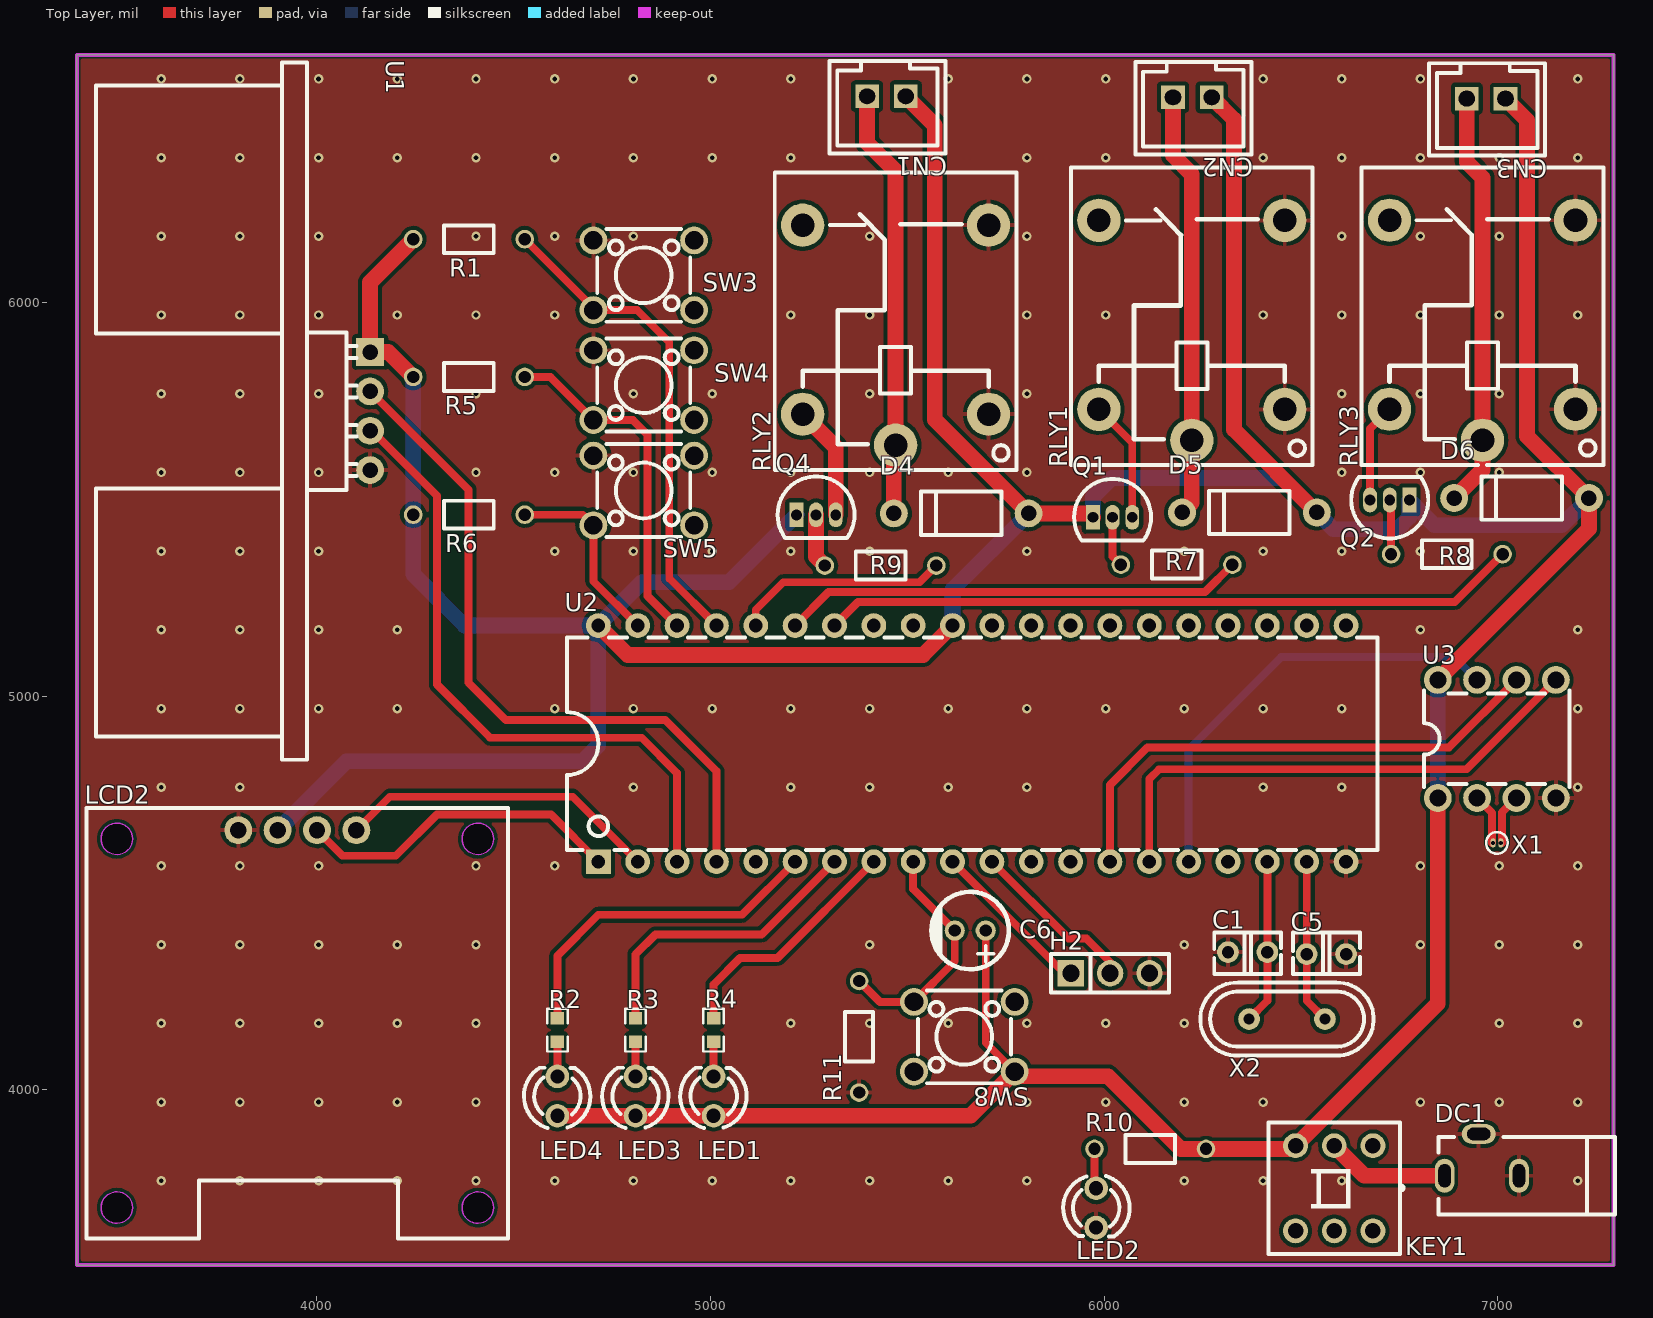
[diagram p0: Top Layer view]
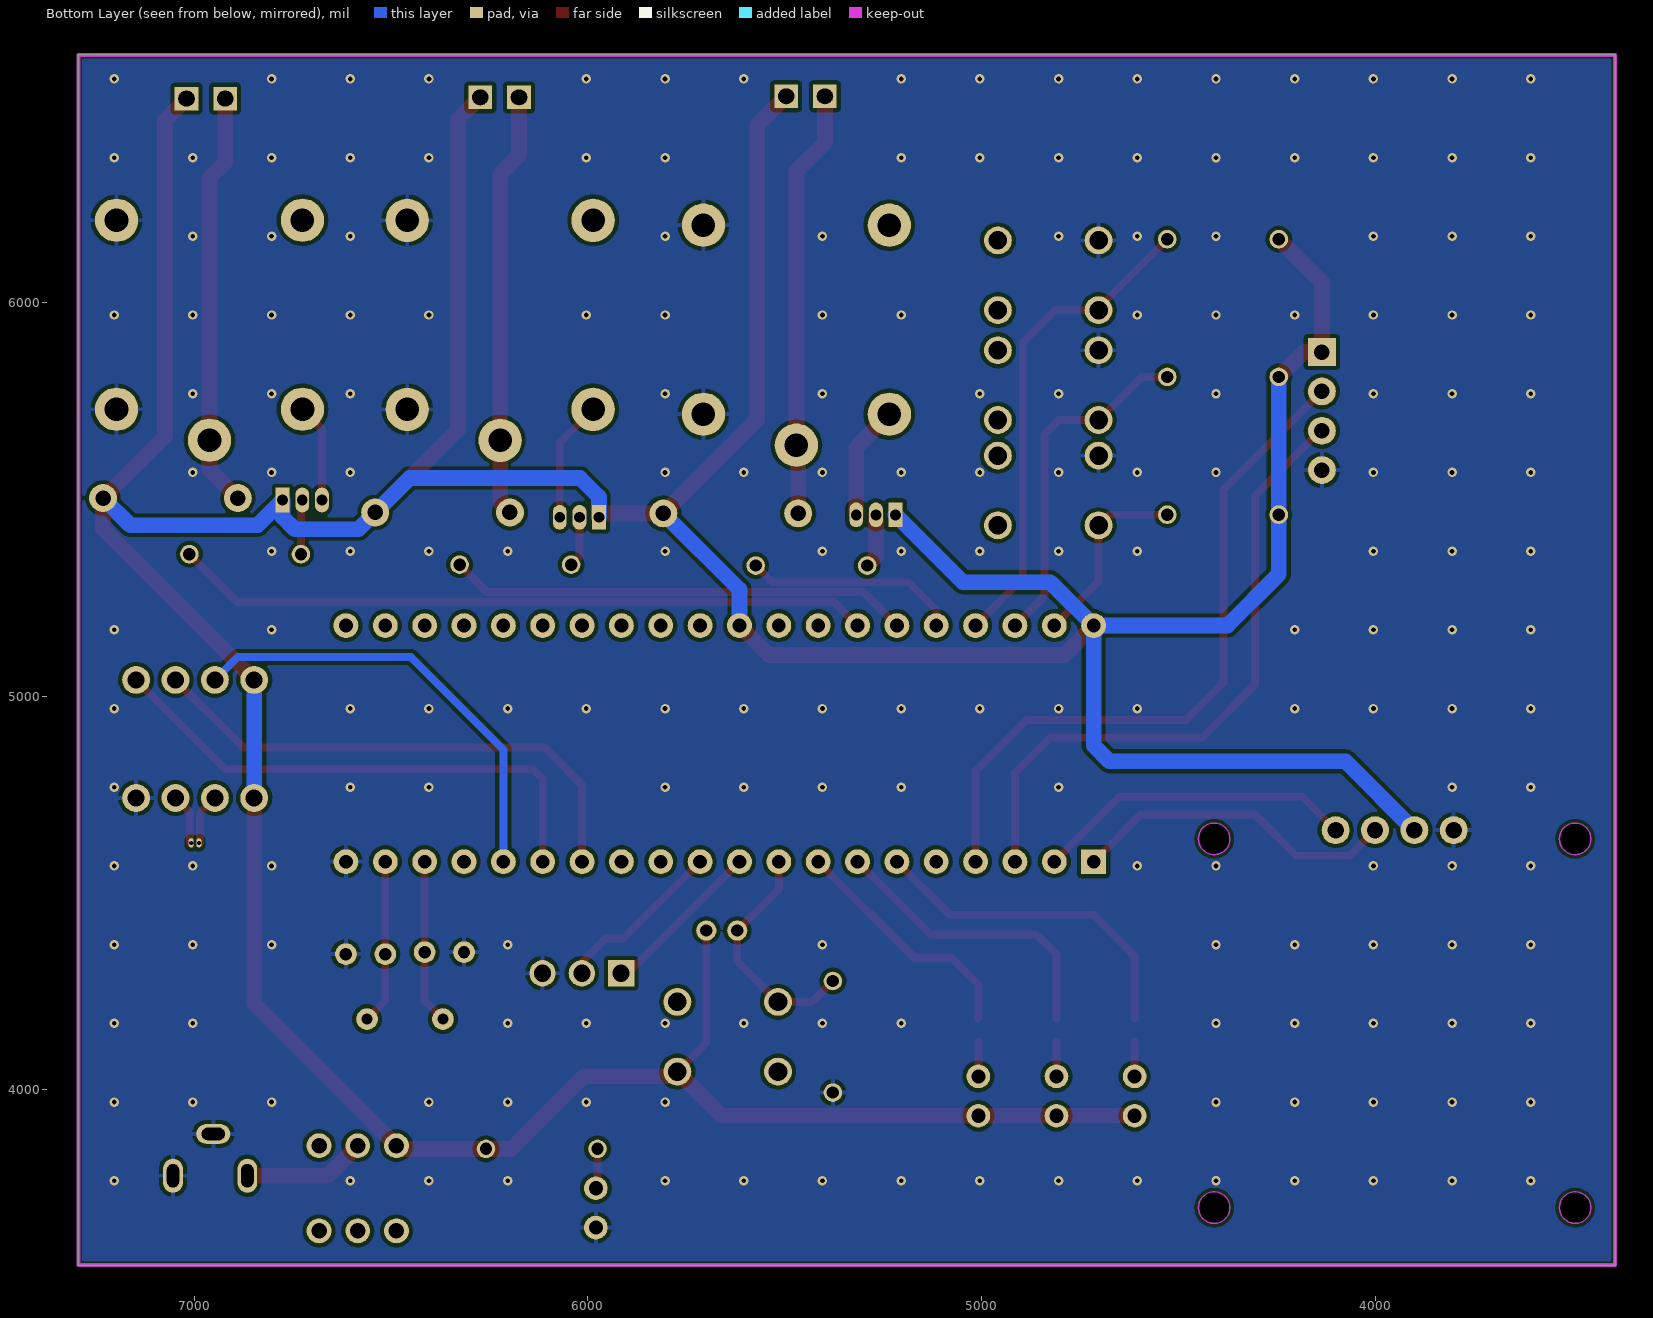
[diagram p1: Bottom Layer view, seen from below]
# Altium PCB MISC52010.pcbdoc
Units mil, origin at the board's own origin, x right, y up, seen from the top; angles counter-clockwise.
Board outline 3905 x 3075 mil, 2 copper layers (Top Layer, Bottom Layer), stack 62.206 mil thick; 43 components, 39 nets, 160 pads, 187 vias.

## Layer stack, top to bottom
Top Solder Mask Layer: solder mask 0.394, Dk 3.3
Top Layer: signal copper 1.379
Dielectric1: surface 59.449, FR4, Dk 4.5
Bottom Layer: signal copper 1.378
Bottom Solder Mask Layer: solder mask 0.394, Dk 3.3

## Board outline
3390,6630 3390,3555 7295,3555 7295,6630

## Design rules (kind name [scope] priority, off if disabled: settings)
BoardOutlineClearance copperThickness2oz_1 [All] p2 off: genericclearance=7.99 ignorepadtopadclearanceinfootprint=FALSE except(0: Arc-SplitContinuation Track-SplitContinuation SMDPad-SplitContinuation THPad-SplitContinuation Via-SplitContinuation Fill-SplitContinuation Region-SplitContinuation Poly-SplitContinuation Text-SplitContinuation Hole-SplitContinuation; 5.98: Arc-CutoutEdge SMDPad-CutoutEdge THPad-CutoutEdge Via-CutoutEdge Fill-CutoutEdge Region-CutoutEdge Text-CutoutEdge; 6.93: Hole-OutlineEdge Hole-CutoutEdge; 10: Poly-OutlineEdge Poly-CutoutEdge; 11.81: Arc-OutlineEdge Track-OutlineEdge SMDPad-OutlineEdge THPad-OutlineEdge Via-OutlineEdge Fill-OutlineEdge Region-OutlineEdge Text-OutlineEdge Track-CutoutEdge)
BoardOutlineClearance copperThickness1oz_1 [All] p4: genericclearance=4.02 ignorepadtopadclearanceinfootprint=FALSE except(0: Arc-SplitContinuation Track-SplitContinuation SMDPad-SplitContinuation THPad-SplitContinuation Via-SplitContinuation Fill-SplitContinuation Region-SplitContinuation Poly-SplitContinuation Text-SplitContinuation Hole-SplitContinuation; 6: SMDPad-CutoutEdge THPad-CutoutEdge Via-CutoutEdge Fill-CutoutEdge Region-CutoutEdge Text-CutoutEdge; 6.93: Hole-OutlineEdge Hole-CutoutEdge; 10: Poly-OutlineEdge Poly-CutoutEdge; 11.8: Arc-OutlineEdge Track-OutlineEdge SMDPad-OutlineEdge THPad-OutlineEdge Via-OutlineEdge Fill-OutlineEdge Region-OutlineEdge Text-OutlineEdge; 11.81: Arc-CutoutEdge Track-CutoutEdge)
Clearance copperThickness2oz [All] p1 off: gap=7.99 ignorepadtopadclearanceinfootprint=FALSE except(5.98: SMDPad-Track SMDPad-SMDPad THPad-Track SMDPad-THPad THPad-THPad Track-Via SMDPad-Via THPad-Via Via-Via Fill-Track Region-Track Fill-SMDPad Region-SMDPad Fill-THPad Region-THPad Fill-Via Region-Via Fill-Fill Fill-Region Region-Region Arc-Track Arc-SMDPad Arc-THPad Arc-Via Fill-Arc Region-Arc Arc-Arc Text-Track SMDPad-Text Text-THPad Text-Via Fill-Text Region-Text Arc-Text Text-Text; 6.93: Hole-Track Hole-SMDPad Hole-THPad Hole-Via Fill-Hole Region-Hole Hole-Arc Hole-Text; 10: Poly-Track Poly-SMDPad Poly-THPad Poly-Via Poly-Fill Poly-Region Poly-Poly Poly-Arc Poly-Text Poly-Hole)
Clearance copperThickness1oz [All] p3: gap=4.02 ignorepadtopadclearanceinfootprint=FALSE except(5.98: SMDPad-Track SMDPad-SMDPad THPad-Track SMDPad-THPad THPad-THPad Track-Via SMDPad-Via THPad-Via Via-Via Fill-Track Region-Track Fill-SMDPad Region-SMDPad Fill-THPad Region-THPad Fill-Via Region-Via Fill-Fill Fill-Region Region-Region; 6: Arc-Track Arc-SMDPad Arc-THPad Arc-Via Fill-Arc Region-Arc Arc-Arc Text-Track SMDPad-Text Text-THPad Text-Via Fill-Text Region-Text Arc-Text Text-Text; 6.93: Hole-Track Hole-SMDPad Hole-THPad Hole-Via Fill-Hole Region-Hole Hole-Arc Hole-Text; 10: Poly-Track Poly-SMDPad Poly-THPad Poly-Via Poly-Fill Poly-Region Poly-Poly Poly-Arc Poly-Text Poly-Hole)
Creepage creepage [All] p1: checkdistance=0 ignoreinternallayers=TRUE applytopolygonpour=TRUE
DiffPairsRouting differentialPair [All] p1: maxlimit=6 minlimit=6 mostfreqgap=6 toplayer_minwidth=5 toplayer_prefwidth=10 toplayer_maxwidth=100 toplayer_mingap=6 toplayer_prefgap=6 toplayer_maxgap=6 bottomlayer_minwidth=5 bottomlayer_prefwidth=10 bottomlayer_maxwidth=100 bottomlayer_mingap=6 bottomlayer_prefgap=6 bottomlayer_maxgap=6 maxuncoupledlength=10
HoleToHoleClearance otherClearance [All] p1: gap=11.81 allowstackedmicrovias=TRUE
Length netLength [All] p1: minlimit=0 maxlimit=0
MatchedLengths netLengthTolerance [All] p1: tolerance=1000
PasteMaskExpansion pasteMaskExpansion [All] p1: expansion=0
PlaneConnect innerPlane [All] p1: planeconnectstyle=Relief reliefexpansion=20 reliefentries=4 reliefconductorwidth=10 reliefairgap=10
PolygonConnect copperRegion [(InNet('GND'))] p1: connectstyle=Relief reliefconductorwidth=10 reliefentries=4 polygonreliefangle="90 Angle" airgapwidth=10 via.connectstyle=Relief via.reliefconductorwidth=10 via.reliefentries=4 via.polygonreliefangle="90 Angle" via.airgapwidth=10
RoutingVias viaSize [All] p1: holewidth=12.01 width=24.02 viastyle="Through Hole" minholewidth=11.81 minwidth=19.68 maxholewidth=248.03 maxwidth=393.7
SolderMaskExpansion solderMaskExpansion [IsVia] p1: expansion=-1000 istentingtop=TRUE
SolderMaskExpansion solderMaskExpansion [All] p2: expansion=2 istentingtop=FALSE
Width copperThickness2oz_2 [All] p1 off: maxlimit=100 minlimit=8 preferedwidth=10
Width copperThickness1oz_2 [All] p2: maxlimit=100 minlimit=5 preferedwidth=10

## Components (designator, comment, footprint, x,y, rotation, side; value= is the part's Value field where it differs from the comment)
C1 "30pF" CAP-TH_L3.8-W2.5-P2.54-D0.50 6365,4350 r0 top
C5 "30pF" CAP-TH_L3.8-W2.5-P2.54-D0.50 6565,4345 r180 top
C6 "10uF" CAP-TH_BD5.0-P2.00-D0.8-FD-10UF50VC110GL 5660,4405 r180 top
CN1 "XH2.54-2PIN-直针" CONN-TH_XH2.54-2P 5447.09,6525.02 r180 top
CN2 "XH2.54-2PIN-直针" CONN-TH_XH2.54-2P 6224.43,6522.35 r180 top
CN3 "XH2.54-2PIN-直针" CONN-TH_XH2.54-2P 6971.03,6518.96 r180 top
D4 "" DO_1N4007 5637.09,5465.02 r0 top
D5 "" DO_1N4007 6369.43,5467.35 r0 top
D6 "" DO_1N4007 7061.03,5503.96 r0 top
DC1 "DC-002" DC-IN-TH_DC-3510 6960,3835 r0 top
H2 "" HDR-TH_3P-P2.54-V-M 6015.53,4296.39 r0 top
KEY1 "无自锁开关 8.5×8.5 无声" SW-TH_6P-L8.5-W8.5-P2.54 6585,3750 r180 top
LCD2 "HS96L03W2C03" OLED-TH_L27.8-W27.2-P2.54_C9900033791 3950,4660 r0 top
LED1 "" LED_TH-3mm 5007.91,3984.24 r90 top
LED2 "" LED_TH-3mm 5980,3700 r270 top
LED3 "" LED_TH-3mm 4809.41,3984.24 r90 top
LED4 "" LED_TH-3mm 4610.91,3984.24 r90 top
Q1 "" S8550P_TO-92 6021.71,5455.16 r0 top
Q2 "" S8550P_TO-92 6726.03,5498.96 r180 top
Q4 "" S8550P_TO-92 5268.28,5461.34 r0 top
R1 "10kΩ" Res_1/8W 4386.23,6164.19 r180 top
R2 "220" R0603 4610.91,4152.03 r90 top
R3 "220" R0603 4809.41,4152.03 r90 top
R4 "220" R0603 5007.91,4152.03 r90 top
R5 "10kΩ" Res_1/8W 4386.23,5814.19 r180 top
R6 "10kΩ" Res_1/8W 4386.23,5464.19 r180 top
R7 "1kΩ" Res_1/8W 6184.43,5332.35 r0 top
R8 "1kΩ" Res_1/8W 6871.03,5358.96 r0 top
R9 "1kΩ" Res_1/8W 5432.09,5330.02 r0 top
R10 "1kΩ" Res_1/8W 6117.48,3847.52 r0 top
R11 "10kΩ" Res_1/8W 5380,4135 r90 top
RLY1 "SRD-05VDC-SL-C" RELAY-TH_SRD-XXVDC-XL-C 6223.04,5930.16 r90 top
RLY2 "SRD-05VDC-SL-C" RELAY-TH_SRD-XXVDC-XL-C 5470.38,5917.82 r90 top
RLY3 "SRD-05VDC-SL-C" RELAY-TH_SRD-XXVDC-XL-C 6961.75,5930.43 r90 top
SW3 "" SW-TH_4P-L6.0-W6.0-P4.50-LS6.5 4830.32,6070.09 r180 top
SW4 "" SW-TH_4P-L6.0-W6.0-P4.50-LS6.5 4830.32,5790.96 r180 top
SW5 "" SW-TH_4P-L6.0-W6.0-P4.50-LS6.5 4830.32,5523.25 r180 top
SW8 "" SW-TH_4P-L6.0-W6.0-P4.50-LS6.5 5645,4135 r180 top
U1 "HC-SR04" TH_HC-SR04V 4135,5725 r270 top
U2 "STC89C52RC-40I-PDIP40" DIP-40_L52.0-W13.7-P2.54-LS15.2-BL 5665,4880 r0 top
U3 "DS1302N(XBLW)" PDIP-8_L9.3-W6.4-P2.54-LS7.6-BL 6998.11,4891.89 r0 top
X1 "32.768kHz" CRYSTAL-TH_BD1.4-P0.45-D0.2 6998.47,4627.72 r180 top
X2 "11.0592MHz" OSC-TH_L11.1-W4.7-P4.88 6465,4180 r180 top

## Footprints (in the part's own frame and the unit in brackets; to place one, negate y for a bottom-side part, rotate by r counter-clockwise, add the part's x,y. Pads: shape width x height; smd on the part's side, far side on the other; paste and mask are expansions set on the pad)
CAP-TH_BD5.0-P2.00-D0.8-FD-10UF50VC110GL [mm]
  round 1.3 hole 0.8: 1(-1,0) 2(1,0)
  silkscreen extent -2.5,-2.5 2.5,2.5
CAP-TH_L3.8-W2.5-P2.54-D0.50 [mm]
  round 1.4 hole 0.8 paste+0 mask+0.05: 1(-1.27,0) 2(1.27,0)
  silkscreen extent -2.16,-1.4 2.16,1.27
CONN-TH_XH2.54-2P [mil]
  rect 60x60 hole 39.37 slot 41.34 at 0 deg paste+0 mask+1.97: 1(-49.22,0) 2(49.21,0)
  silkscreen extent -150,-90 145,145
CRYSTAL-TH_BD1.4-P0.45-D0.2 [mm]
  oval 0.32x0.6 hole 0.27 paste+0 mask+0.05: 1(-0.25,0) 2(0.25,0)
  silkscreen extent -0.7,-0.7 0.7,0.7
DC-IN-TH_DC-3510 [mm]
  oval 1.27x2.2 hole 0.8 slot 1.5 at 90 deg: 1(-2.4,-1.35) 2(2.4,-1.35)
  oval 2.2x1.27 hole 0.8 slot 1.5 at 0 deg: 3(-0.2,1.35)
  silkscreen extent -2.8,-3.85 8.6,1.15
DIP-40_L52.0-W13.7-P2.54-LS15.2-BL [mil]
  rect 63x63 hole 35: 1(-950,-300)
  round 63 hole 35: 2(-850,-300) 3(-750,-300) 4(-650,-300) 5(-550,-300) 6(-450,-300) 7(-350,-300) 8(-250,-300) 9(-150,-300) 10(-50,-300) 11(50,-300) 12(150,-300) 13(250,-300) 14(350,-300) 15(450,-300) 16(550,-300) 17(650,-300) 18(750,-300) 19(850,-300) 20(950,-300) 21(950,300) 22(850,300) 23(750,300) 24(650,300) 25(550,300) 26(450,300) 27(350,300) 28(250,300) 29(150,300) 30(50,300) 31(-50,300) 32(-150,300) 33(-250,300) 34(-350,300) 35(-450,300) 36(-550,300) 37(-650,300) 38(-750,300) 39(-850,300) 40(-950,300)
  silkscreen extent -1030,-270 1030,270
DO_1N4007 [mm]
  round 1.8 hole 1 paste+0 mask+0.051: 1(-4.35,0) 2(4.35,0)
  silkscreen extent -2.6,-1.4 2.6,1.4
HDR-TH_3P-P2.54-V-M [mm]
  rect 1.7x1.7 hole 1.1: 1(-2.54,0)
  round 1.7 hole 1.1: 2(0,0) 3(2.54,0)
  silkscreen extent -3.81,-1.25 3.81,1.25
LED_TH-3mm [mil]
  round 60 hole 36 paste+0 mask+2: 1(-50,0) 2(50,0)
  silkscreen extent -81,-84 72,85
OLED-TH_L27.8-W27.2-P2.54_C9900033791 [mm]
  round 1.8 hole 1.05 paste+0 mask+0.05: 1(-3.81,0) 2(-1.27,0) 3(1.27,0) 4(3.81,0)
  Board Outline Layer circle w0.003: c-11.65,-0.56 r1.016
  Board Outline Layer circle w0.003: c11.65,-0.56 r1.016
  Board Outline Layer circle w0.003: c-11.65,-24.36 r1.016
  Board Outline Layer circle w0.003: c11.65,-24.36 r1.016
  Board Outline Layer region: -10.634,-0.56 -10.735,-1.001 -11.016,-1.354 -11.424,-1.551 -11.876,-1.551 -12.283,-1.354 -12.565,-1.001 -12.666,-0.56 -12.666,-0.56 -12.565,-0.119 -12.283,0.234 -11.876,0.431 -11.424,0.431 -11.016,0.234 -10.735,-0.119 -10.634,-0.56
  Board Outline Layer region: -10.634,-0.56 -10.643,-0.698 -10.672,-0.834 -10.718,-0.965 -10.782,-1.088 -10.862,-1.201 -10.956,-1.303 -11.064,-1.39 -11.183,-1.462 -11.31,-1.517 -11.443,-1.555 -11.581,-1.574 -11.719,-1.574 -11.857,-1.555 -11.99,-1.517 -12.117,-1.462 -12.236,-1.39 -12.343,-1.303 -12.438,-1.201 -12.518,-1.088 -12.582,-0.965 -12.628,-0.834 -12.656,-0.698 -12.666,-0.56 -12.656,-0.422 -12.628,-0.286 -12.582,-0.155 -12.518,-0.032 -12.438,0.081 -12.343,0.183 -12.236,0.27 -12.117,0.342 -11.99,0.397 -11.857,0.435 -11.719,0.454 -11.581,0.454 -11.443,0.435 -11.31,0.397 -11.183,0.342 -11.064,0.27 -10.956,0.183 -10.862,0.081 -10.782,-0.032 -10.718,-0.155 -10.672,-0.286 -10.643,-0.422
  Board Outline Layer region: 12.666,-0.56 12.565,-1.001 12.283,-1.354 11.876,-1.551 11.424,-1.551 11.017,-1.354 10.735,-1.001 10.634,-0.56 10.634,-0.56 10.735,-0.119 11.017,0.234 11.424,0.431 11.876,0.431 12.283,0.234 12.565,-0.119 12.666,-0.56
  Board Outline Layer region: 12.666,-0.56 12.657,-0.698 12.628,-0.834 12.582,-0.965 12.518,-1.088 12.438,-1.201 12.343,-1.303 12.236,-1.39 12.117,-1.462 11.99,-1.517 11.857,-1.555 11.719,-1.574 11.581,-1.574 11.443,-1.555 11.31,-1.517 11.183,-1.462 11.064,-1.39 10.957,-1.303 10.862,-1.201 10.782,-1.088 10.718,-0.965 10.672,-0.834 10.643,-0.698 10.634,-0.56 10.643,-0.422 10.672,-0.286 10.718,-0.155 10.782,-0.032 10.862,0.081 10.957,0.183 11.064,0.27 11.183,0.342 11.31,0.397 11.443,0.435 11.581,0.454 11.719,0.454 11.857,0.435 11.99,0.397 12.117,0.342 12.236,0.27 12.343,0.183 12.438,0.081 12.518,-0.032 12.582,-0.155 12.628,-0.286 12.657,-0.422
  Board Outline Layer region: -10.634,-24.36 -10.735,-24.801 -11.016,-25.154 -11.424,-25.35 -11.876,-25.35 -12.283,-25.154 -12.565,-24.801 -12.666,-24.36 -12.666,-24.36 -12.565,-23.919 -12.283,-23.566 -11.876,-23.369 -11.424,-23.369 -11.016,-23.566 -10.735,-23.919 -10.634,-24.36
  Board Outline Layer region: -10.634,-24.36 -10.643,-24.498 -10.672,-24.634 -10.718,-24.765 -10.782,-24.888 -10.862,-25.001 -10.956,-25.102 -11.064,-25.19 -11.183,-25.262 -11.31,-25.317 -11.443,-25.355 -11.581,-25.374 -11.719,-25.374 -11.857,-25.355 -11.99,-25.317 -12.117,-25.262 -12.236,-25.19 -12.343,-25.102 -12.438,-25.001 -12.518,-24.888 -12.582,-24.765 -12.628,-24.634 -12.656,-24.498 -12.666,-24.36 -12.656,-24.222 -12.628,-24.086 -12.582,-23.955 -12.518,-23.832 -12.438,-23.719 -12.343,-23.617 -12.236,-23.53 -12.117,-23.458 -11.99,-23.403 -11.857,-23.365 -11.719,-23.346 -11.581,-23.346 -11.443,-23.365 -11.31,-23.403 -11.183,-23.458 -11.064,-23.53 -10.956,-23.617 -10.862,-23.719 -10.782,-23.832 -10.718,-23.955 -10.672,-24.086 -10.643,-24.222
  Board Outline Layer region: 12.666,-24.36 12.565,-24.801 12.283,-25.154 11.876,-25.35 11.424,-25.35 11.017,-25.154 10.735,-24.801 10.634,-24.36 10.634,-24.36 10.735,-23.919 11.017,-23.566 11.424,-23.369 11.876,-23.369 12.283,-23.566 12.565,-23.919 12.666,-24.36
  Board Outline Layer region: 12.666,-24.36 12.657,-24.498 12.628,-24.634 12.582,-24.765 12.518,-24.888 12.438,-25.001 12.343,-25.102 12.236,-25.19 12.117,-25.262 11.99,-25.317 11.857,-25.355 11.719,-25.374 11.581,-25.374 11.443,-25.355 11.31,-25.317 11.183,-25.262 11.064,-25.19 10.957,-25.102 10.862,-25.001 10.782,-24.888 10.718,-24.765 10.672,-24.634 10.643,-24.498 10.634,-24.36 10.643,-24.222 10.672,-24.086 10.718,-23.955 10.782,-23.832 10.862,-23.719 10.957,-23.617 11.064,-23.53 11.183,-23.458 11.31,-23.403 11.443,-23.365 11.581,-23.346 11.719,-23.346 11.857,-23.365 11.99,-23.403 12.117,-23.458 12.236,-23.53 12.343,-23.617 12.438,-23.719 12.518,-23.832 12.582,-23.955 12.628,-24.086 12.657,-24.222
  Multi-Layer board cut-out: -10.634,-0.56 -10.735,-1.001 -11.016,-1.354 -11.424,-1.551 -11.876,-1.551 -12.283,-1.354 -12.565,-1.001 -12.666,-0.56 -12.666,-0.56 -12.565,-0.119 -12.283,0.234 -11.876,0.431 -11.424,0.431 -11.016,0.234 -10.735,-0.119 -10.634,-0.56
  Multi-Layer board cut-out: 12.666,-0.56 12.565,-1.001 12.283,-1.354 11.876,-1.551 11.424,-1.551 11.017,-1.354 10.735,-1.001 10.634,-0.56 10.634,-0.56 10.735,-0.119 11.017,0.234 11.424,0.431 11.876,0.431 12.283,0.234 12.565,-0.119 12.666,-0.56
  Multi-Layer board cut-out: -10.634,-24.36 -10.735,-24.801 -11.016,-25.154 -11.424,-25.35 -11.876,-25.35 -12.283,-25.154 -12.565,-24.801 -12.666,-24.36 -12.666,-24.36 -12.565,-23.919 -12.283,-23.566 -11.876,-23.369 -11.424,-23.369 -11.016,-23.566 -10.735,-23.919 -10.634,-24.36
  Multi-Layer board cut-out: 12.666,-24.36 12.565,-24.801 12.283,-25.154 11.876,-25.35 11.424,-25.35 11.017,-25.154 10.735,-24.801 10.634,-24.36 10.634,-24.36 10.735,-23.919 11.017,-23.566 11.424,-23.369 11.876,-23.369 12.283,-23.566 12.565,-23.919 12.666,-24.36
  silkscreen extent -13.6,-26.36 13.6,1.44
OSC-TH_L11.1-W4.7-P4.88 [mm]
  round 1.4 hole 0.7: 1(-2.45,0) 2(2.45,0)
  silkscreen extent -5.59,-2.35 5.6,2.35
PDIP-8_L9.3-W6.4-P2.54-LS7.6-BL [mm]
  round 1.8 hole 1.1: 1(-3.81,-3.81) 2(-1.27,-3.81) 3(1.27,-3.81) 4(3.81,-3.81) 5(3.81,3.81) 6(1.27,3.81) 7(-1.27,3.81) 8(-3.81,3.81)
  silkscreen extent -4.7,-3.11 4.7,3.11
R0603 [mil]
  rect 31.75x34.02 smd paste-3937.01 mask+2: 1(-29.66,0) 2(29.66,0)
  silkscreen extent -55,-26 55,26
RELAY-TH_SRD-XXVDC-XL-C [mil]
  round 110 hole 60: 1(-200.79,-236.22) 2(279.53,-236.2) 3(279.53,236.2) 4(-200.79,236.22) 5(-279.53,0)
  silkscreen extent -342,-307 413,307
Res_1/8W [mil]
  round 47.2 hole 31.5 paste+0 mask+2: 1(-141.7,2.48) 2(141.7,2.48)
  silkscreen extent -63,-33 63,38
S8550P_TO-92 [mm]
  rect 0.9x1.6 hole 0.7 paste+0 mask+0.051: 1(-1.27,0)
  oval 0.9x1.6 hole 0.7 paste+0 mask+0.051: 2(0,0) 3(1.27,0)
  silkscreen extent -2.48,-1.5 2.48,2.48
SW-TH_4P-L6.0-W6.0-P4.50-LS6.5 [mm]
  round 1.8 hole 1.2: 1(-3.25,2.25) 2(3.25,2.25) 3(-3.25,-2.25) 4(3.25,-2.25)
  silkscreen extent -3,-3 3,3
SW-TH_6P-L8.5-W8.5-P2.54 [mm]
  round 1.6 hole 1: 1(-2.5,-2.75) 2(0,-2.75) 3(2.5,-2.75) 4(-2.5,2.75) 5(0,2.75) 6(2.5,2.75)
  silkscreen extent -4.47,-4.25 4.25,4.25
TH_HC-SR04V [mm]
  rect 1.8x1.8 hole 1.001: 1(-3.81,0)
  round 1.8 hole 1.001: 2(-1.27,0) 3(1.27,0) 4(3.81,0)
  silkscreen extent -22.5,-17.7 22.5,-0.89

## Via types
v1: diameter 24.02, hole 12, Top Layer to Bottom Layer, 187 vias

## Nets (pads, with @x,y where several pads share a name; then routed paths per layer and width w, separated by ;. In a path a pad name is that pad's centre, name@x,y a point inside that pad or via, vN(x,y) a via of type N, cw(c..) or ccw(c..) an arc to the next point about the centre after c; other vN are vias at no path point)
$1N19: LED1.2 R4.1 | length 88.1
  Top Layer w20: LED1.2 R4.1
$1N20: R4.2 U2.8 | length 622.6
  Top Layer w20: R4.2 5007.91,4267.91 5075,4335 5170,4335 U2.8
$1N23: LED3.2 R3.1 | length 88.1
  Top Layer w20: LED3.2 R3.1
$1N24: R3.2 U2.7 | length 765.9
  Top Layer w20: R3.2 4809.41,4344.41 4860,4395 5130,4395 U2.7
$1N25: LED4.2 R2.1 | length 88.1
  Top Layer w20: LED4.2 R2.1
$1N26: R2.2 U2.6 | length 862.3
  Top Layer w20: R2.2 4610.91,4340.91 4715,4445 5080,4445 U2.6
$1N30: U1.2 U2.4 | length 1796.8
  Top Layer w20: U1.2 4385,5525 4385,5035 4480,4940 4885,4940 5015,4810 U2.4
$1N34: U1.3 U2.3 | length 1646.5
  Top Layer w20: U1.3 4140,5675 4305,5510 4305,5030 4440,4895 4825,4895 4915,4805 U2.3
$1N36: LCD2.4 U2.2 | length 818.6
  Top Layer w20: LCD2.4 4185,4745 4650,4745 U2.2
$1N37: LCD2.3 U2.1 | length 835.1
  Top Layer w20: LCD2.3 4065,4595 4200,4595 4305,4700 4595,4700 U2.1
$1N43: R1.1 SW3.2 U2.37 | length 1248.6
  Top Layer w20: R1.1 4702.37,5987.27 SW3.2 4813.49,5981.51 4895,5900 4895,5300 U2.37
$1N44: R5.1 SW4.2 U2.38 | length 888.9
  Top Layer w20: R5.1 4593.04,5811.71 SW4.2 4802.62,5702.38 4840,5665 4840,5255 U2.38
$1N45: R6.1 SW5.2 U2.39 | length 487
  Top Layer w20: R6.1 4675.33,5461.71 SW5.2 4702.37,5292.63 U2.39
$1N52: Q4.2 R9.1 | length 138
  Top Layer w40: Q4.2 5268.28,5354.61 R9.1
$1N53: Q4.3 RLY2.4 | length 290.5
  Top Layer w40: RLY2.4 5318.28,5632.92 Q4.3
$1N57: CN1.2 D4.1 RLY2.5 | length 1091.9
  Top Layer w40: CN1.2 5397.88,6407.12 5470.38,6334.62 RLY2.5 5465.83,5633.75 D4.1
$1N60: CN2.2 D5.1 RLY1.5 | length 1085.1
  Top Layer w40: CN2.2 6175.21,6374.79 6223.04,6326.96 RLY1.5 6223.04,5492.23 D5.1
$1N64: Q1.2 R7.1 | length 129
  Top Layer w20: Q1.2 6021.71,5355.85 R7.1
$1N65: Q1.3 RLY1.4 | length 309.4
  Top Layer w20: RLY1.4 6071.71,5644.48 Q1.3
$1N68: CN3.2 D6.1 RLY3.5 | length 1061.4
  Top Layer w40: D6.1 6961.75,5575.93 RLY3.5 6961.75,6318.25 6921.82,6358.18 CN3.2
$1N72: Q2.2 R8.1 | length 138.9
  Top Layer w20: Q2.2 6729.33,5495.66 R8.1
$1N73: Q2.3 RLY3.4 | length 251.2
  Top Layer w20: Q2.3 6676.03,5680.15 RLY3.4
$1N79: U3.2 X1.2 | length 129.9
  Top Layer w20: U3.2 6986.03,4703.97 X1.2@6986.03,4627.72
$1N80: U3.3 X1.1 | length 129.6
  Top Layer w20: X1.1@7010.91,4627.72 7010.91,4704.68 U3.3
$1N83: U2.16 U3.7 | length 1139.5
  Bottom Layer w20: U2.16 6215,4865 6450,5100 6890,5100 U3.7
$1N84: U2.14 U3.6 | length 1338.7
  Top Layer w20: U2.14 6015,4775 6110,4870 6876.23,4870 U3.6
$1N85: U2.15 U3.5 | length 1347.4
  Top Layer w20: U2.15 6115,4790 6140,4815 6921.23,4815 U3.5
$1N99: LED2.1 R10.1 | length 101.7
  Top Layer w20: R10.1 5975.78,3754.22 LED2.1
$1N101: DC1.1 KEY1.2 | length 312.2
  Top Layer w40: KEY1.2 6661.43,3781.85 DC1.1
+5V: C6.1 CN1.1 CN2.1 CN3.1 D4.2 D5.2 D6.2 KEY1.3 LCD2.2 LED1.1 LED3.1 LED4.1 Q1.1 Q2.1 Q4.1 R1.2 R5.2 R6.2 R10.2 SW8.1 U1.1 U2.31 U2.40 U3.1 U3.8 | length 14122.2
  Top Layer w20: C6.1 5699.37,4120 SW8.1
  Top Layer w40: R5.2 4181.24,5875 U1.1 4135,6052.18 R1.2 ; LED4.1 LED3.1 LED1.1 5660.77,3934.24 SW8.1 5784.37,4035 6010,4035 6195,3850 R10.2 6478.31,3850 KEY1.3 6848.11,4219.81 U3.1 ; U2.40 4790,5105 5540,5105 U2.31 ; CN1.1 5570,6451.32 5570,5703.37 D4.2 5961.86,5465.02 Q1.1 ; CN2.1 6330,6466 6330,5678.04 D5.2 ; U3.8 7232.29,5426.07 D6.2 7075,5661.25 7075,6464.21 CN3.1
  Bottom Layer w40: LCD2.2 4075,4835 4675,4835 4715,4875 U2.40 ; R5.2 R6.2 4244.53,5310.47 4375,5180 U2.40 ; Q4.1 5046.94,5290 4825,5290 U2.40 ; U2.31 5615,5271.66 D4.2 ; Q1.1 5971.71,5506.71 6020,5555 6453.04,5555 D5.2 6583.04,5425 6745,5425 6776.03,5456.03 Q2.1 6839.99,5435 7163.34,5435 D6.2 ; U3.1 U3.8
GND: C1.1 C5.1 DC1.2 DC1.3 H2.3 LCD2.1 LED2.2 R11.1 RLY1.1 RLY1.2 RLY2.1 RLY2.2 RLY3.1 RLY3.2 SW3.4 SW4.4 SW5.4 U1.4 U2.20 U3.4
  other v1: 3604.1,3769.1 3804.1,3769.1 4004.1,3769.1 4204.1,3769.1 4404.1,3769.1 4604.1,3769.1 4804.1,3769.1 5004.1,3769.1 5204.1,3769.1 5404.1,3769.1 5604.1,3769.1 5804.1,3769.1 6204.1,3769.1 6404.1,3769.1 6604.1,3769.1 7204.1,3769.1 3604.1,3969.1 3804.1,3969.1 4004.1,3969.1 4204.1,3969.1 4404.1,3969.1 5804.1,3969.1 6004.1,3969.1 6204.1,3969.1 6404.1,3969.1 6804.1,3969.1 7004.1,3969.1 7204.1,3969.1 3604.1,4169.1 3804.1,4169.1 4004.1,4169.1 4204.1,4169.1 4404.1,4169.1 5204.1,4169.1 5404.1,4169.1 5604.1,4169.1 5804.1,4169.1 6004.1,4169.1 6204.1,4169.1 7004.1,4169.1 7204.1,4169.1 3604.1,4369.1 3804.1,4369.1 4004.1,4369.1 4204.1,4369.1 4404.1,4369.1 5404.1,4369.1 6204.1,4369.1 6804.1,4369.1 7004.1,4369.1 7204.1,4369.1 3604.1,4569.1 3804.1,4569.1 4004.1,4569.1 4404.1,4569.1 4604.1,4569.1 6804.1,4569.1 7004.1,4569.1 7204.1,4569.1 3604.1,4769.1 3804.1,4769.1 4804.1,4769.1 5204.1,4769.1 5404.1,4769.1 5604.1,4769.1 5804.1,4769.1 6404.1,4769.1 6604.1,4769.1 7204.1,4769.1 3604.1,4969.1 3804.1,4969.1 4004.1,4969.1 4204.1,4969.1 4604.1,4969.1 4804.1,4969.1 5004.1,4969.1 5204.1,4969.1 5404.1,4969.1 5604.1,4969.1 5804.1,4969.1 6004.1,4969.1 6204.1,4969.1 6404.1,4969.1 6604.1,4969.1 7204.1,4969.1 3604.1,5169.1 3804.1,5169.1 4004.1,5169.1 4204.1,5169.1 6804.1,5169.1 7204.1,5169.1 3604.1,5369.1 3804.1,5369.1 4004.1,5369.1 4604.1,5369.1 4804.1,5369.1 5004.1,5369.1 5204.1,5369.1 5404.1,5369.1 5804.1,5369.1 6204.1,5369.1 6404.1,5369.1 6604.1,5369.1 6804.1,5369.1 3604.1,5569.1 3804.1,5569.1 4004.1,5569.1 4404.1,5569.1 4604.1,5569.1 4804.1,5569.1 5004.1,5569.1 5204.1,5569.1 5404.1,5569.1 5604.1,5569.1 5804.1,5569.1 6604.1,5569.1 6804.1,5569.1 7004.1,5569.1 3604.1,5769.1 3804.1,5769.1 4004.1,5769.1 4404.1,5769.1 4804.1,5769.1 5004.1,5769.1 5404.1,5769.1 5804.1,5769.1 6604.1,5769.1 6804.1,5769.1 7004.1,5769.1 3604.1,5969.1 3804.1,5969.1 4004.1,5969.1 4204.1,5969.1 4404.1,5969.1 4604.1,5969.1 5204.1,5969.1 5404.1,5969.1 5804.1,5969.1 6004.1,5969.1 6404.1,5969.1 6604.1,5969.1 6804.1,5969.1 7004.1,5969.1 7204.1,5969.1 3604.1,6169.1 3804.1,6169.1 4004.1,6169.1 4404.1,6169.1 4604.1,6169.1 4804.1,6169.1 5404.1,6169.1 5804.1,6169.1 6604.1,6169.1 6804.1,6169.1 7004.1,6169.1 3604.1,6369.1 3804.1,6369.1 4004.1,6369.1 4204.1,6369.1 4404.1,6369.1 4604.1,6369.1 4804.1,6369.1 5004.1,6369.1 5204.1,6369.1 5804.1,6369.1 6004.1,6369.1 6404.1,6369.1 6604.1,6369.1 6804.1,6369.1 7004.1,6369.1 7204.1,6369.1 3604.1,6569.1 3804.1,6569.1 4004.1,6569.1 4204.1,6569.1 4404.1,6569.1 4604.1,6569.1 4804.1,6569.1 5004.1,6569.1 5204.1,6569.1 5604.1,6569.1 5804.1,6569.1 6004.1,6569.1 6404.1,6569.1 6604.1,6569.1 6804.1,6569.1 7204.1,6569.1
P03: R9.2 U2.36 | length 545.4
  Top Layer w20: U2.36 5115,5220 5185,5290 5531.3,5290 R9.2
P04: R7.2 U2.35 | length 1175.3
  Top Layer w20: U2.35 5300,5265 6256.3,5265 R7.2
P05: R8.2 U2.34 | length 1772.9
  Top Layer w20: U2.34 5375,5240 6891.3,5240 R8.2
P30: H2.1 U2.10 | length 418
  Top Layer w20: U2.10 5898.61,4296.39 H2.1
P31: H2.2 U2.11 | length 434.5
  Top Layer w20: U2.11 5910,4385 5955,4385 6015.53,4324.47 H2.2
RST: C6.2 R11.2 SW8.4 U2.9 | length 604.6
  Top Layer w20: R11.2 5430.64,4223.58 SW8.4 5620.63,4327.16 C6.2 5515,4510.63 U2.9
X1: C5.2 U2.19 X2.1 | length 419.2
  Top Layer w20: U2.19 C5.2 6515,4226.45 X2.1
X2: C1.2 U2.18 X2.2 | length 419.2
  Top Layer w20: X2.2 6415,4226.45 C1.2 U2.18
pads on no net: KEY1.1 KEY1.4 KEY1.5 KEY1.6 RLY1.3 RLY2.3 RLY3.3 SW3.1 SW3.3 SW4.1 SW4.3 SW5.1 SW5.3 SW8.2 SW8.3 U2.5 U2.12 U2.13 U2.17 U2.21 U2.22 U2.23 U2.24 U2.25 U2.26 U2.27 U2.28 U2.29 U2.30 U2.32 U2.33

## Polygon pours and split planes (outlines as drawn)
GND on Top Layer (solid, remove dead copper, pour order 0): 3000,7160 3000,3000 7780,3000 7780,7160
GND on Bottom Layer (solid, remove dead copper, pour order 2): 3310,6810 3310,3300 7530,3300 7530,6810

## Keep-outs
Board Outline Layer:
  the board outline again, w10